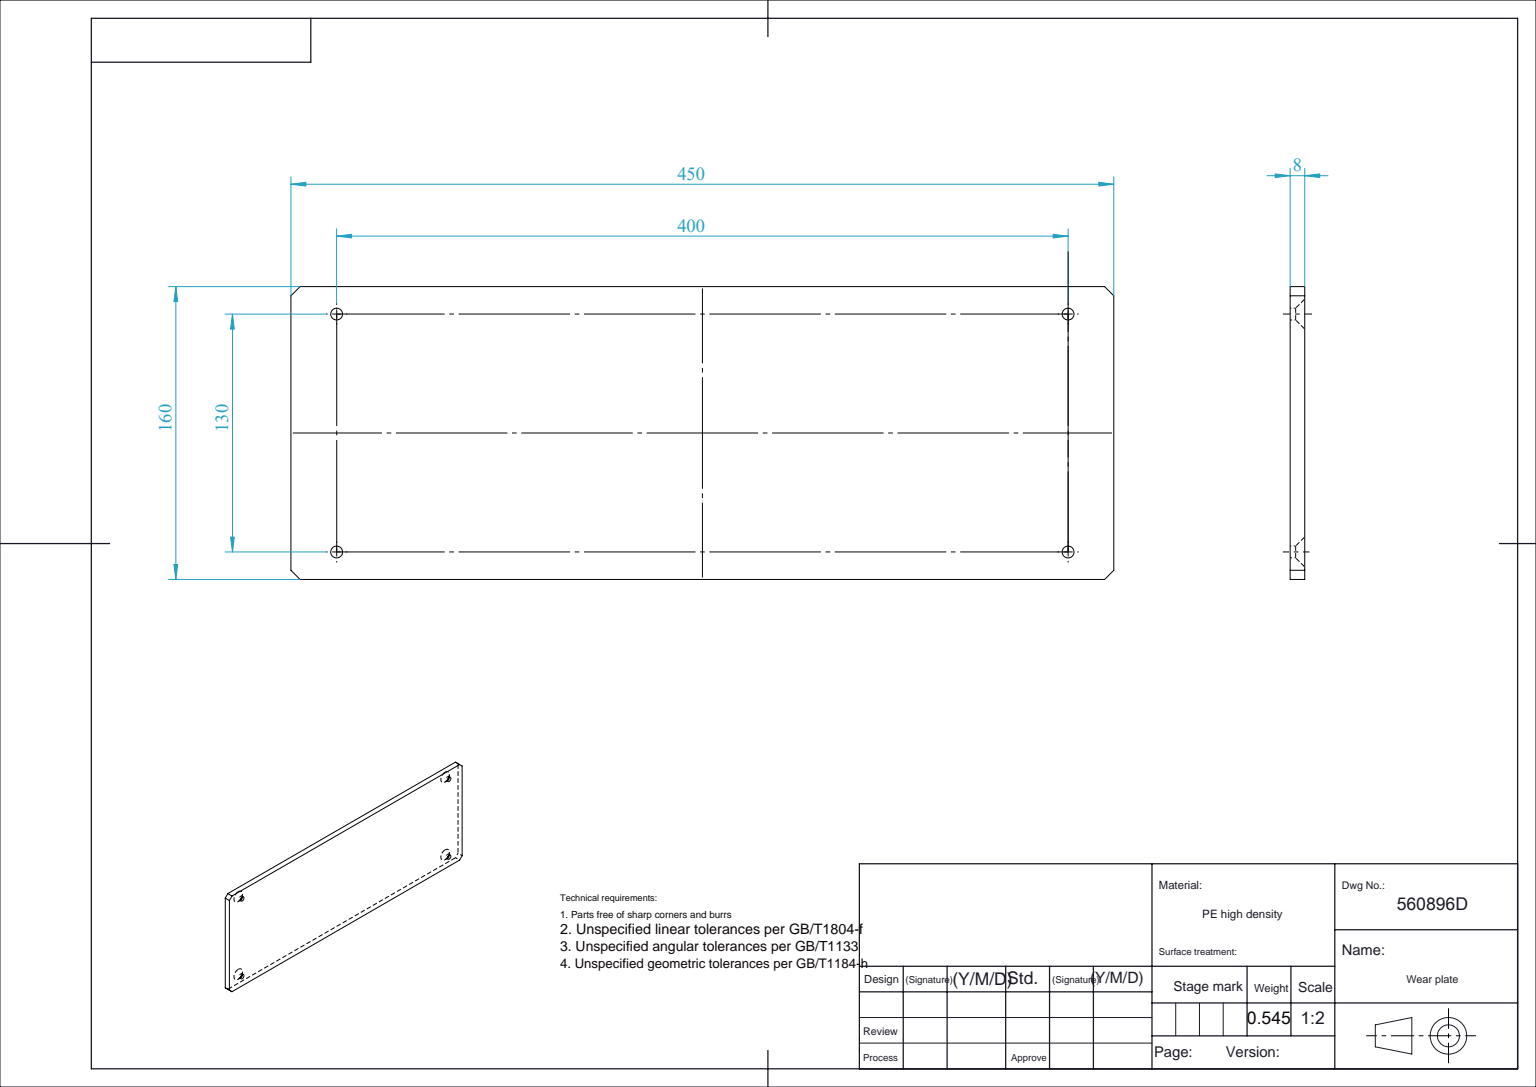
from build123d import *

# Parameters (mm, degrees)
SKETCH1_W                    = 450
SKETCH1_H                    = 160
BOSS_EXTRUDE1_DEPTH          = 8
SKETCH15_R                   = 3.25
CUT_EXTRUDE5_DEPTH           = 8
SKETCH16_R                   = 8.25
CUT_EXTRUDE6_DEPTH           = 5
CUT_EXTRUDE6_DRAFT           = -45
CUT_EXTRUDE6_PROFILE_2_DEPTH = 5
CUT_EXTRUDE6_PROFILE_2_DRAFT = -45
CUT_EXTRUDE6_PROFILE_3_DEPTH = 5
CUT_EXTRUDE6_PROFILE_3_DRAFT = -45
CUT_EXTRUDE6_PROFILE_4_DEPTH = 5
CUT_EXTRUDE6_PROFILE_4_DRAFT = -45
CHAMFER1_SIZE                = 5


with BuildPart() as part:
    # Sketch1 → Boss-Extrude1 (new body)
    with BuildSketch(Plane(origin=(0, 0, 0), x_dir=(1, 0, 0), z_dir=(0, 1, 0))):
        Rectangle(SKETCH1_W, SKETCH1_H)
    extrude(amount=BOSS_EXTRUDE1_DEPTH)

    # Sketch15 → Cut-Extrude5 (cut)
    with BuildSketch(Plane.XZ):
        with Locations(Location((-200, 65, 0), (0, 0, 270))):
            Circle(SKETCH15_R)
        with Locations(Location((-200, -65, 0), (0, 0, 270))):
            Circle(SKETCH15_R)
        with Locations(Location((200, 65, 0), (0, 0, 270))):
            Circle(SKETCH15_R)
        with Locations(Location((200, -65, 0), (0, 0, 270))):
            Circle(SKETCH15_R)
    extrude(amount=-CUT_EXTRUDE5_DEPTH, mode=Mode.SUBTRACT)


with BuildPart() as cut_extrude6_tool:
    # Sketch16 → Cut-Extrude6 (with draft: the straight prism first)
    with BuildSketch(Plane.XZ):
        with Locations((-200, 65)):
            Circle(SKETCH16_R)
    extrude(amount=-CUT_EXTRUDE6_DEPTH)
    # Cut-Extrude6: the draft: its side faces are tilted about the plane it starts from
    cut_extrude6_sides = [cut_extrude6_tool.faces().sort_by_distance(p)[0] for p in [
        (-208.25, 2.5, 65),
    ]]
    draft(cut_extrude6_sides, Plane.XZ, CUT_EXTRUDE6_DRAFT)


with BuildPart() as part_1:
    add(part.part)

    # Cut-Extrude6: cut by cut_extrude6_tool
    add(cut_extrude6_tool.part, mode=Mode.SUBTRACT)


with BuildPart() as cut_extrude6_profile_2_tool:
    # Sketch16 → Cut-Extrude6 profile 2 (with draft: the straight prism first)
    with BuildSketch(Plane.XZ):
        with Locations((-200, -65)):
            Circle(SKETCH16_R)
    extrude(amount=-CUT_EXTRUDE6_PROFILE_2_DEPTH)
    # Cut-Extrude6 profile 2: the draft: its side faces are tilted about the plane it starts from
    cut_extrude6_profile_2_sides = [cut_extrude6_profile_2_tool.faces().sort_by_distance(p)[0] for p in [
        (-208.25, 2.5, -65),
    ]]
    draft(cut_extrude6_profile_2_sides, Plane.XZ, CUT_EXTRUDE6_PROFILE_2_DRAFT)


with BuildPart() as part_2:
    add(part_1.part)

    # Cut-Extrude6 profile 2: cut by cut_extrude6_profile_2_tool
    add(cut_extrude6_profile_2_tool.part, mode=Mode.SUBTRACT)


with BuildPart() as cut_extrude6_profile_3_tool:
    # Sketch16 → Cut-Extrude6 profile 3 (with draft: the straight prism first)
    with BuildSketch(Plane.XZ):
        with Locations((200, 65)):
            Circle(SKETCH16_R)
    extrude(amount=-CUT_EXTRUDE6_PROFILE_3_DEPTH)
    # Cut-Extrude6 profile 3: the draft: its side faces are tilted about the plane it starts from
    cut_extrude6_profile_3_sides = [cut_extrude6_profile_3_tool.faces().sort_by_distance(p)[0] for p in [
        (191.75, 2.5, 65),
    ]]
    draft(cut_extrude6_profile_3_sides, Plane.XZ, CUT_EXTRUDE6_PROFILE_3_DRAFT)


with BuildPart() as part_3:
    add(part_2.part)

    # Cut-Extrude6 profile 3: cut by cut_extrude6_profile_3_tool
    add(cut_extrude6_profile_3_tool.part, mode=Mode.SUBTRACT)


with BuildPart() as cut_extrude6_profile_4_tool:
    # Sketch16 → Cut-Extrude6 profile 4 (with draft: the straight prism first)
    with BuildSketch(Plane.XZ):
        with Locations((200, -65)):
            Circle(SKETCH16_R)
    extrude(amount=-CUT_EXTRUDE6_PROFILE_4_DEPTH)
    # Cut-Extrude6 profile 4: the draft: its side faces are tilted about the plane it starts from
    cut_extrude6_profile_4_sides = [cut_extrude6_profile_4_tool.faces().sort_by_distance(p)[0] for p in [
        (191.75, 2.5, -65),
    ]]
    draft(cut_extrude6_profile_4_sides, Plane.XZ, CUT_EXTRUDE6_PROFILE_4_DRAFT)


with BuildPart() as part_4:
    add(part_3.part)

    # Cut-Extrude6 profile 4: cut by cut_extrude6_profile_4_tool
    add(cut_extrude6_profile_4_tool.part, mode=Mode.SUBTRACT)

    # Chamfer1
    chamfer1_edges = [part_4.edges().sort_by_distance(p)[0] for p in [
        (225, 4, 80),
        (-225, 4, 80),
        (-225, 4, -80),
        (225, 4, -80),
    ]]
    chamfer(chamfer1_edges, length=CHAMFER1_SIZE)


solid = part_4.part
